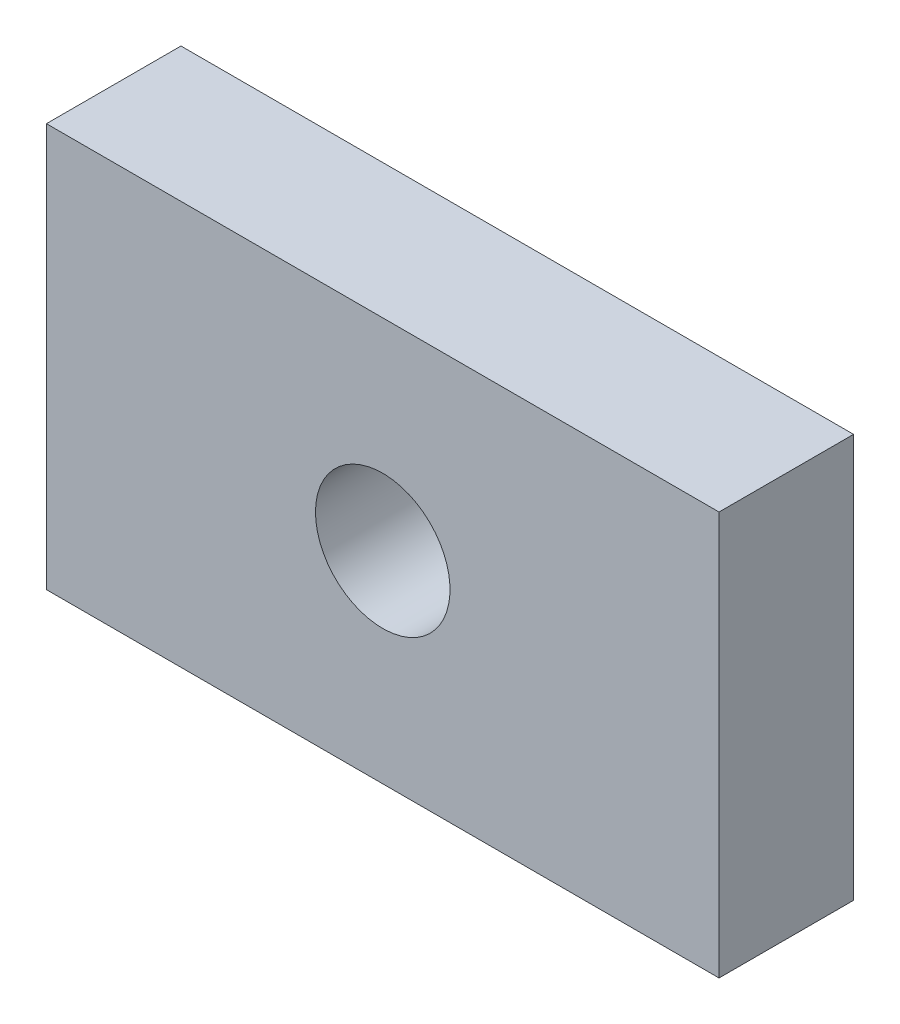
SolidWorks part; units mm, degrees
ref_plane "Front Plane" through (0, 0, 0) normal (0, 0, 1) x (1, 0, 0)
ref_plane "Top Plane" through (0, 0, 0) normal (0, 1, 0) x (1, 0, 0)
ref_plane "Right Plane" through (0, 0, 0) normal (1, 0, 0) x (0, 0, -1)
ref_plane "Plane1" through (0, 0, 5) normal (0, 0, 1) x (1, 0, 0)
sketch "Sketch1" plane through (0, 0, 5) normal (0, 0, 1) x (1, 0, 0)
  line L0 (-25, 15) -> (-25, -15)
  line L1 (-25, -15) -> (25, -15)
  line L2 (25, -15) -> (25, 15)
  line L3 (25, 15) -> (-25, 15)
  circle A0 centre (0, 0) radius 5
extrude "Boss-Extrude1" add sketch "Sketch1" against normal blind 10
